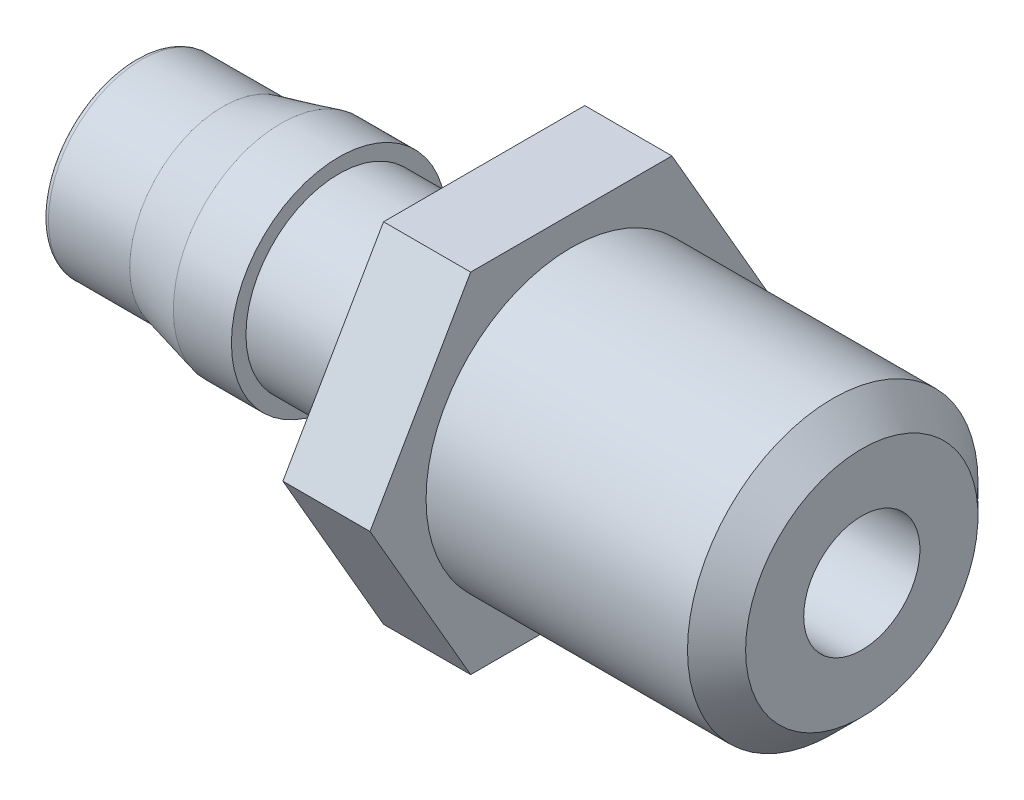
from build123d import *

# Parameters (mm, degrees)
SKETCH2_OUTSIDE_W  = 14.568
SKETCH2_OUTSIDE_H  = 14.568
CUT_EXTRUDE3_DEPTH = 10
FILLET1_R          = 0.1
CHAMFER1_SIZE      = 0.5


with BuildPart() as part:
    # Sketch1 → Revolve1 (revolve)
    with BuildSketch(Plane.XY, mode=Mode.PRIVATE) as revolve1_sk:
        Polygon((0, 1), (12.5, 1), (12.5, 2.5), (7.5, 2.5), (7.5, 4.5), (6, 4.5), (6, 1.6), (3.5, 1.6), (3.5, 1.85), (2.5, 1.85), (1.5, 1.6), (0, 1.6), align=None)
    revolve(revolve1_sk.sketch.rotate(Axis((0, 0, 0), (1, 0, 0)), 90), axis=Axis((0, 0, 0), (1, 0, 0)))

    # Sketch2 outside → Cut-Extrude3 (cut)
    with BuildSketch(Plane(origin=(7.5, 0, 0), x_dir=(0, 0, -1), z_dir=(1, 0, 0))):
        Rectangle(SKETCH2_OUTSIDE_W, SKETCH2_OUTSIDE_H)
        Polygon((1.732050808, -3), (3.464101615, 0), (1.732050808, 3), (-1.732050808, 3), (-3.464101615, 0), (-1.732050808, -3), align=None, mode=Mode.SUBTRACT)
    extrude(amount=-CUT_EXTRUDE3_DEPTH, mode=Mode.SUBTRACT)

    # Fillet1
    fillet1_edges = [part.edges().sort_by_distance(p)[0] for p in [
        (0, 0, -1.6),
    ]]
    fillet(fillet1_edges, radius=FILLET1_R)

    # Chamfer1
    chamfer1_edges = [part.edges().sort_by_distance(p)[0] for p in [
        (12.5, 0, -2.5),
    ]]
    chamfer(chamfer1_edges, length=CHAMFER1_SIZE)


solid = part.part
